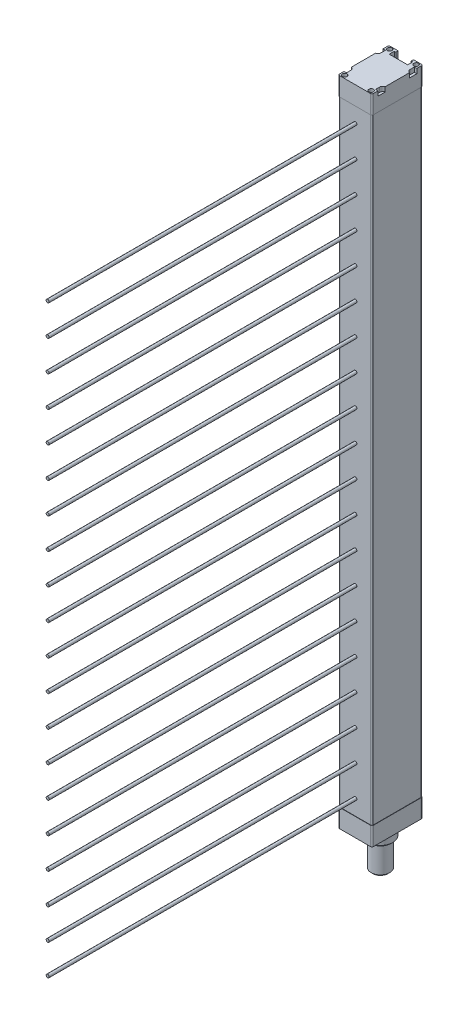
SolidWorks part; units mm, degrees
material "A6061"
ref_plane "前基準面" through (0, 0, 0) normal (0, 0, 1) x (1, 0, 0)
ref_plane "上基準面" through (0, 0, 0) normal (0, 1, 0) x (1, 0, 0)
ref_plane "右基準面" through (0, 0, 0) normal (1, 0, 0) x (0, 0, -1)
sketch "草圖1" plane through (0, 0, 0) normal (0, 1, 0) x (1, 0, 0)
  line L0 (-11, 0) -> (11, 0) construction
  line L1 (-10, 16.5) -> (-5, 16.5)
  line L2 (-11, 15.5) -> (-11, -15.5)
  line L3 (-10, -16.5) -> (10, -16.5)
  line L4 (11, 15.5) -> (11, -15.5)
  line L5 (0, 0) -> (0, 16.4415) construction
  line L6 (-5, 15) -> (-6, 15)
  line L7 (-5, 16.5) -> (-5, 15)
  line L9 (5, 16.5) -> (5, 15)
  line L10 (5, 16.5) -> (10, 16.5)
  line L11 (6, 15) -> (5, 15)
  line L12 (6, 15) -> (6, 11.7)
  line L13 (6, 11.7) -> (-6, 11.7)
  line L14 (-6, 15) -> (-6, 11.7)
  line L15 (6, 15) -> (-6, 11.7) construction
  line L16 (6, 11.7) -> (-6, 15) construction
  circle A0 centre (-8.6, 14.6) radius 1.5
  circle A1 centre (8.6, 14.6) radius 1.5
  circle A2 centre (8.6, -14.6) radius 1.5
  circle A3 centre (-8.6, -14.6) radius 1.5
  arc A4 (-10, 16.5) -> (-11, 15.5) centre (-10, 15.5) ccw
  arc A5 (11, 15.5) -> (10, 16.5) centre (10, 15.5) ccw
  arc A6 (11, -15.5) -> (10, -16.5) centre (10, -15.5) cw
  arc A7 (-11, -15.5) -> (-10, -16.5) centre (-10, -15.5) ccw
  point P21 (0, 13.35)
  dimension "D6" = 3
  dimension "D10" = 1
  dimension "D1" = 22
  dimension "D2" = 33
  dimension "D3" = 10
  dimension "D4" = 1.5
  dimension "D5" = 4.8
  dimension "D7" = 2.4
  dimension "D8" = 3.3
  dimension "D9" = 12
  dimension "D11" = 1.9
extrude "伸長1" add sketch "草圖1" along normal blind 12
sketch "草圖2" plane through (0, 12, 0) normal (0, 1, 0) x (1, 0, 0)
  line L0 (0, 0) -> (0, 14.9784) construction
  line L1 (-14.2, 12.65) -> (-9.4, 12.65)
  line L2 (-14.2, 12.65) -> (-14.2, 7.85)
  line L3 (-14.2, 7.85) -> (-11.4, 7.85)
  line L4 (-9.4, 12.65) -> (-9.4, 9.85)
  line L5 (0, 0) -> (15.7654, 0) construction
  line L6 (9.4, 12.65) -> (9.4, 9.85)
  line L7 (14.2, 7.85) -> (11.4, 7.85)
  line L8 (14.2, 12.65) -> (14.2, 7.85)
  line L9 (14.2, 12.65) -> (9.4, 12.65)
  line L10 (14.2, -12.65) -> (9.4, -12.65)
  line L11 (14.2, -12.65) -> (14.2, -7.85)
  line L12 (14.2, -7.85) -> (11.4, -7.85)
  line L13 (9.4, -12.65) -> (9.4, -9.85)
  line L14 (-9.4, -12.65) -> (-9.4, -9.85)
  line L15 (-14.2, -7.85) -> (-11.4, -7.85)
  line L16 (-14.2, -12.65) -> (-14.2, -7.85)
  line L17 (-14.2, -12.65) -> (-9.4, -12.65)
  arc A0 (-9.4, 9.85) -> (-11.4, 7.85) centre (-11.4, 9.85) cw
  arc A1 (9.4, 9.85) -> (11.4, 7.85) centre (11.4, 9.85) ccw
  arc A2 (9.4, -9.85) -> (11.4, -7.85) centre (11.4, -9.85) cw
  arc A3 (-9.4, -9.85) -> (-11.4, -7.85) centre (-11.4, -9.85) ccw
  point P17 (-15.7654, 0)
  dimension "D1" = 2
  dimension "D2" = 4.8
  dimension "D3" = 4.8
extrude "伸長2" cut sketch "草圖2" against normal blind 3
sketch "草圖3" plane through (0, 0, 0) normal (0, -1, 0) x (1, 0, 0)
  line L48 (-5.2, -16.3) -> (-5.2, -15.2)
  line L49 (-5.2, -15.2) -> (-6.2, -15.2)
  line L50 (-6.2, -15.2) -> (-6.2, -11.5)
  line L51 (-6.2, -11.5) -> (6.2, -11.5)
  line L52 (6.2, -11.5) -> (6.2, -15.2)
  line L53 (6.2, -15.2) -> (5.2, -15.2)
  line L54 (5.2, -15.2) -> (5.2, -16.3)
  line L55 (5.2, -16.3) -> (10, -16.3)
  line L56 (10.8, -15.5) -> (10.8, 15.5)
  line L57 (10, 16.3) -> (-10, 16.3)
  line L58 (-10.8, 15.5) -> (-10.8, -15.5)
  line L59 (-10, -16.3) -> (-5.2, -16.3)
  line L60 (-5.2, -16.3) -> (-5.2, -15.2)
  line L61 (-5.2, -15.2) -> (-6.2, -15.2)
  line L62 (-6.2, -15.2) -> (-6.2, -11.5)
  line L63 (-6.2, -11.5) -> (6.2, -11.5)
  line L64 (6.2, -11.5) -> (6.2, -15.2)
  line L65 (6.2, -15.2) -> (5.2, -15.2)
  line L66 (5.2, -15.2) -> (5.2, -16.3)
  line L67 (5.2, -16.3) -> (10, -16.3)
  line L68 (10.8, -15.5) -> (10.8, 15.5)
  line L69 (10, 16.3) -> (-10, 16.3)
  line L70 (-10.8, 15.5) -> (-10.8, -15.5)
  line L71 (-10, -16.3) -> (-5.2, -16.3)
  arc A12 (10, -16.3) -> (10.8, -15.5) centre (10, -15.5) ccw
  arc A13 (10.8, 15.5) -> (10, 16.3) centre (10, 15.5) ccw
  arc A14 (-10, 16.3) -> (-10.8, 15.5) centre (-10, 15.5) ccw
  arc A15 (-10.8, -15.5) -> (-10, -16.3) centre (-10, -15.5) ccw
  arc A16 (10, -16.3) -> (10.8, -15.5) centre (10, -15.5) ccw
  arc A17 (10.8, 15.5) -> (10, 16.3) centre (10, 15.5) ccw
  arc A18 (-10, 16.3) -> (-10.8, 15.5) centre (-10, 15.5) ccw
  arc A19 (-10.8, -15.5) -> (-10, -16.3) centre (-10, -15.5) ccw
  dimension "D2" = 21.6
  dimension "D3" = 32.6
  dimension "D1" = 0.2
extrude "伸長3" add sketch "草圖3" along normal blind 400
ref_plane "平面1" through (0, -200, 0) normal (0, 1, 0) x (-1, 0, 0)
mirror "鏡射1" about plane through (0, -200, 0) normal (0, 1, 0) of "伸長1"
sketch "草圖4" plane through (0, 0, 0) normal (1, 0, 0) x (0, 0, -1)
  line L0 (0, -412) -> (0, -251.8701) construction
  line L1 (-15.5, -412) -> (15.5, -412) construction
  line L2 (8, -412) -> (8, -419)
  line L3 (8, -419) -> (7, -419)
  line L4 (7, -419) -> (7, -420)
  line L5 (7, -420) -> (6, -420)
  line L6 (6, -420) -> (6, -437)
  line L7 (5, -438) -> (0, -438)
  line L8 (0, -438) -> (0, -412)
  line L9 (6, -437) -> (5, -438)
  line L10 (0, -412) -> (8, -412)
  point P12 (6, -438)
  dimension "D1" = 7
  dimension "D2" = 19
  dimension "D3" = 1
  dimension "D4" = 16
  dimension "D5" = 1
  dimension "D7" = 1
revolve "旋轉1" add sketch "草圖4" angle 360 about L0
sketch "草圖5" plane through (0, 0, 16.3) normal (0, 0, 1) x (1, 0, 0)
  line L0 (0, 12) -> (0, -438) construction
  line L1 (-10, 12) -> (10, 12) construction
  line L2 (-5, -438) -> (5, -438) construction
  line L3 (-10, 0) -> (10, 0) construction
  circle A0 centre (0, -10) radius 1
  dimension "D1" = 2
  dimension "D2" = 10
extrude "伸長4" add sketch "草圖5" along normal blind 200
pattern_linear "阵列(线性)1" count 20 spacing 20 along (0, -1, 0) of "伸長4"
